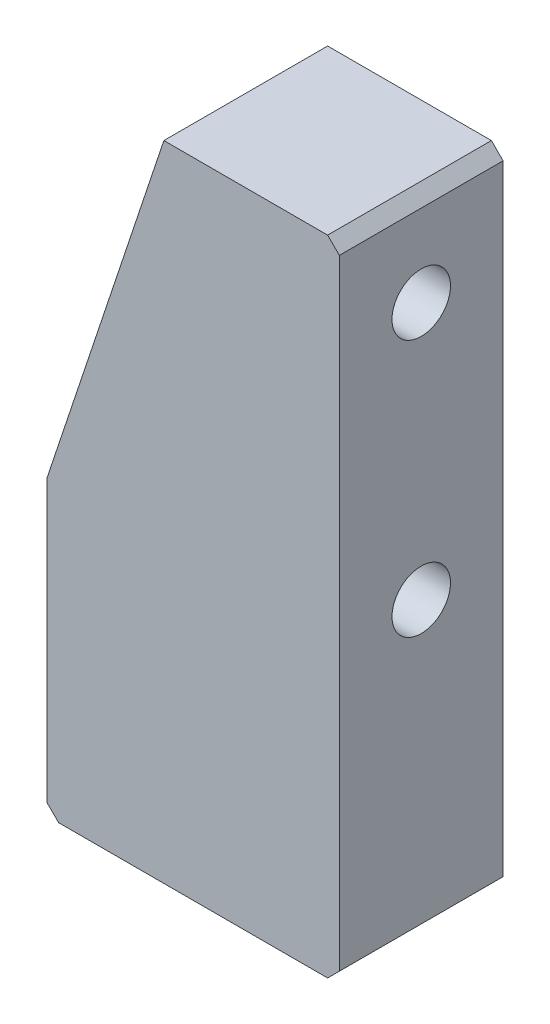
SolidWorks part; units mm, degrees
material "AL6061"
ref_plane "Front Plane" through (0, 0, 0) normal (0, 0, 1) x (1, 0, 0)
ref_plane "Top Plane" through (0, 0, 0) normal (0, 1, 0) x (1, 0, 0)
ref_plane "Right Plane" through (0, 0, 0) normal (1, 0, 0) x (0, 0, -1)
sketch "Sketch6" plane through (0, 0, 0) normal (0, 0, 1) x (1, 0, 0)
  line L14 (0, 0) -> (0, 55)
  line L15 (0, 55) -> (-15, 55)
  line L17 (-25, 25) -> (-25, 0)
  line L18 (-25, 0) -> (0, 0)
  line L19 (-25, 25) -> (-15, 55)
  dimension "D1" = 55
  dimension "D2" = 15
  dimension "D3" = 25
  dimension "D4" = 25
extrude "Boss-Extrude2" add sketch "Sketch6" along normal mid plane 14
hole_wizard "M6 Tapped Hole1" positions "Sketch9" profile "Sketch10" tap size "M6" standard "GB"
sketch "Sketch9" plane through (0, 0, 0) normal (1, 0, 0) x (0, 0, -1)
  line L0 (0, 0) -> (0, 62.3045) construction
  line L1 (-7, 55) -> (7, 55) construction
  line L2 (-7, 0) -> (7, 0) construction
  point P6 (0, 47)
  point P8 (0, 25)
  dimension "D1" = 8
  dimension "D2" = 25
  dimension "D3" = 22
sketch "Sketch10" plane through (0, 25, 0) normal (0, 1, 0) x (0, 0, -1)
  line L0 (0, 0) -> (0, 16.5022)
  line L1 (0, 16.5022) -> (2.5, 15)
  line L2 (2.5, 15) -> (2.5, 0)
  line L5 (2.5, 0) -> (0, 0)
  line L10 (0, 16.5022) -> (-2.5, 15) construction
  line L11 (0, -6.35) -> (0, 107.95) construction
  dimension "螺纹孔钻头直径" = 5
  dimension "螺纹孔钻头深度" = 15
  dimension "导头角度" = 118
cosmetic thread "Cosmetic Thread1" parameters "D1"=12, "D2"=6
cosmetic thread "Cosmetic Thread2" parameters "D1"=12, "D2"=6
hole_wizard "M6 Tapped Hole2" positions "Sketch11" profile "Sketch12" tap size "M6" standard "GB"
sketch "Sketch11" plane through (0, 0, 0) normal (0, -1, 0) x (-1, 0, 0)
  line L0 (0, 0) -> (34.0325, 0) construction
  line L1 (0, -7) -> (0, 7) construction
  point P6 (16, 0)
  dimension "D1" = 16
sketch "Sketch12" plane through (-16, 0, 0) normal (1, 0, 0) x (0, 0, -1)
  line L0 (0, 0) -> (0, 16.5022)
  line L1 (0, 16.5022) -> (2.5, 15)
  line L2 (2.5, 15) -> (2.5, 0)
  line L5 (2.5, 0) -> (0, 0)
  line L10 (0, 16.5022) -> (-2.5, 15) construction
  line L11 (0, -6.35) -> (0, 107.95) construction
  dimension "螺纹孔钻头直径" = 5
  dimension "螺纹孔钻头深度" = 15
  dimension "导头角度" = 118
cosmetic thread "Cosmetic Thread3" parameters "D1"=12, "D2"=6
chamfer "Chamfer1" distance 1 angle 45 3 edges at (-25, 0, 0) (0, 0, 0) (0, 55, 0)
